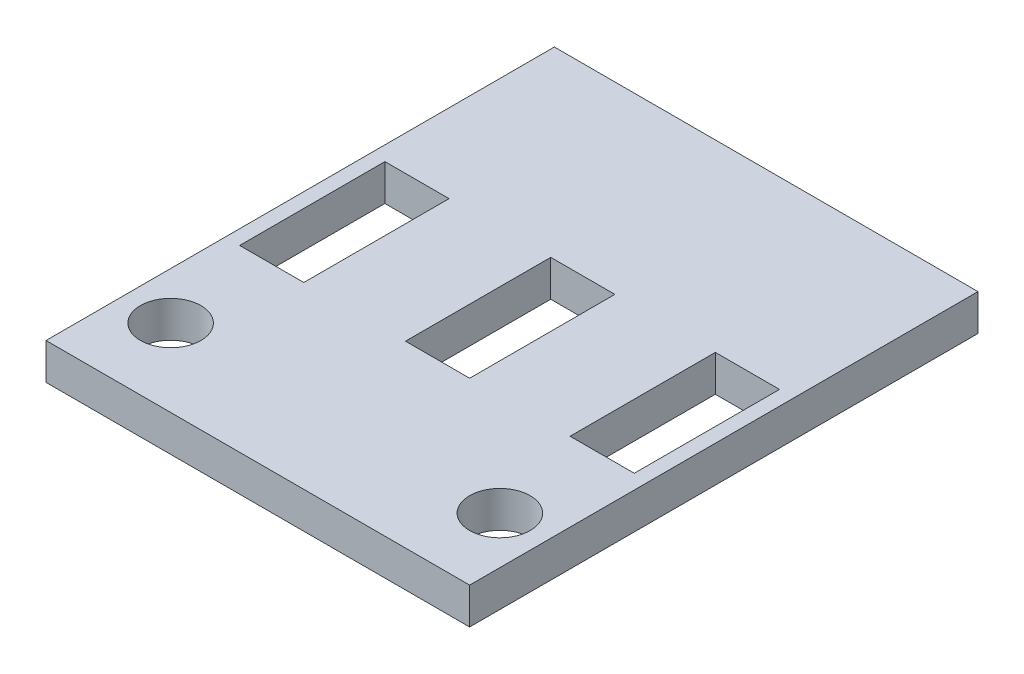
from build123d import *

# Parameters (mm, degrees)
SKETCH1_W           = 350
SKETCH1_H           = 420
SKETCH1_R           = 25
SKETCH1_W_2         = 53
SKETCH1_H_2         = 120
BOSS_EXTRUDE1_DEPTH = 30


with BuildPart() as part:
    # Sketch1 → Boss-Extrude1 (new body)
    with BuildSketch(Plane(origin=(0, 0, 0), x_dir=(1, 0, 0), z_dir=(0, 1, 0))):
        with Locations((175, 210)):
            Rectangle(SKETCH1_W, SKETCH1_H)
        with Locations(Location((311, 64, 0), (0, 0, 270))):
            Circle(SKETCH1_R, mode=Mode.SUBTRACT)
        with Locations(Location((39, 64, 0), (0, 0, 270))):
            Circle(SKETCH1_R, mode=Mode.SUBTRACT)
        with Locations((175.5, 208)):
            Rectangle(SKETCH1_W_2, SKETCH1_H_2, mode=Mode.SUBTRACT)
        with Locations((311.5, 208)):
            Rectangle(SKETCH1_W_2, SKETCH1_H_2, mode=Mode.SUBTRACT)
        with Locations((38.5, 208)):
            Rectangle(SKETCH1_W_2, SKETCH1_H_2, mode=Mode.SUBTRACT)
    extrude(amount=BOSS_EXTRUDE1_DEPTH)


solid = part.part
